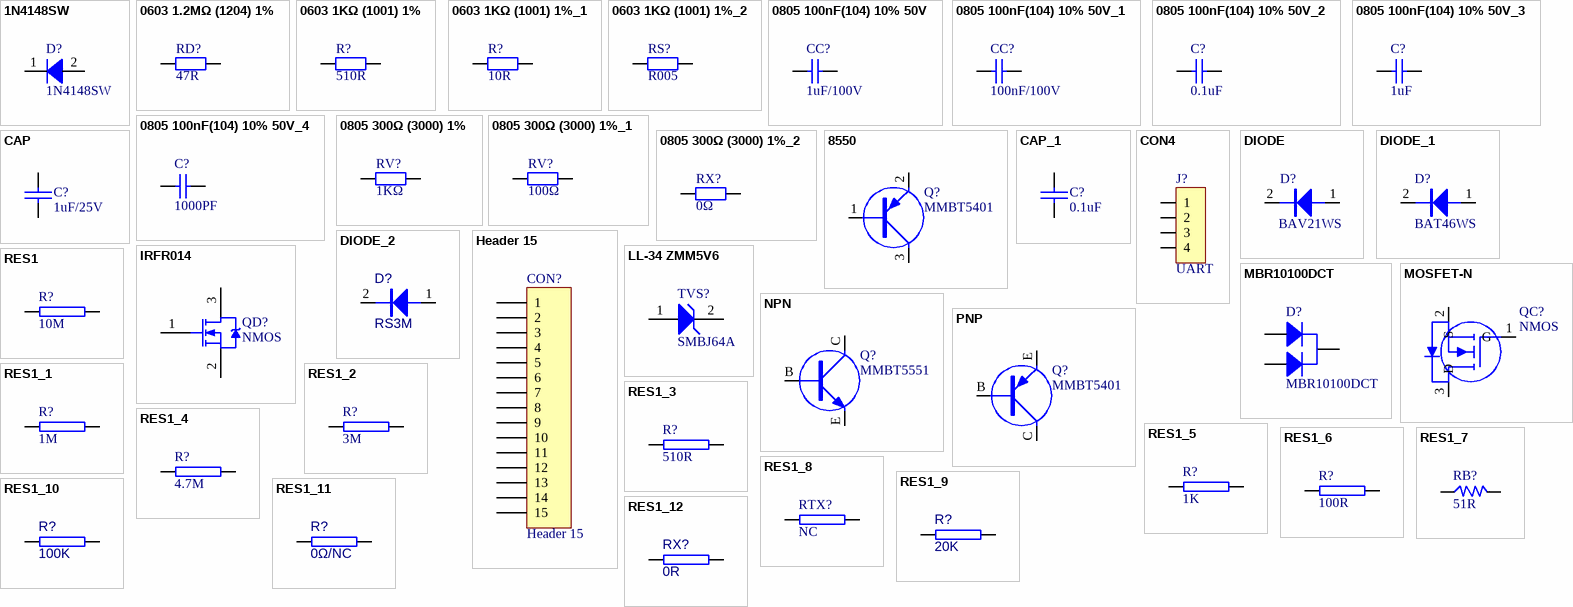
[diagram p0: symbols 1N4148SW to RES1_12]
# Altium schematic symbol library MISC84412-4.SchLib: 47 symbols
Pins are listed as number, name and electrical type; pins without a type are passive.


## 1N4148SW
designator D?
SMD diode
footprint SOD123 (SMD diode)
footprint SOD323 (SMD diode)
pins: 1 A, 2    

## 0603 1.2MΩ (1204) 1%
designator RD?, comment 47R
SMD resistor
footprint RES0603 (CAP0402)
footprint R0603A (SMD resistor)
footprint R0603Ap (SMD resistor)
pins: 1, 2
2 alternate drawings of the same symbol

## 0603 1KΩ (1001) 1%
designator R?, comment 510R
SMD resistor
footprint RES0603 (CAP0402)
footprint R0603A (SMD resistor)
footprint R0402L (SMD resistor)
footprint R0402A (SMD resistor)
pins: 1, 2
2 alternate drawings of the same symbol

## 0603 1KΩ (1001) 1%_1
designator R?, comment 10R
SMD resistor
footprint RES0603 (CAP0402)
footprint R0603A (SMD resistor)
footprint C0402A (SMD capacitor)
footprint R0402A (SMD resistor)
pins: 1, 2
2 alternate drawings of the same symbol

## 0603 1KΩ (1001) 1%_2
designator RS?, comment R005
SMD resistor
footprint 2512
footprint R2512L (SMD resistor)
pins: 1, 2
2 alternate drawings of the same symbol

## 0805 100nF(104) 10% 50V
designator CC?, comment 1uF/100V
SMD capacitor
footprint CAP0805
footprint C0805L (SMD capacitor)
pins: 1, 2
2 alternate drawings of the same symbol

## 0805 100nF(104) 10% 50V_1
designator CC?, comment 100nF/100V
SMD capacitor
footprint CAP0805
footprint C0603L (SMD J capacitor)
footprint C0805A (SMD capacitor)
footprint C0603A (SMD capacitor)
pins: 1, 2
2 alternate drawings of the same symbol

## 0805 100nF(104) 10% 50V_2
designator C?, comment 0.1uF
SMD capacitor
footprint CAP0603 (CAP0402)
footprint C0603A (SMD capacitor)
footprint C0402L (SMD resistor)
footprint C0402A (SMD capacitor)
pins: 1, 2
2 alternate drawings of the same symbol

## 0805 100nF(104) 10% 50V_3
designator C?, comment 1uF
SMD capacitor
footprint CAP0603 (CAP0402)
footprint C0603A (SMD capacitor)
footprint C0402L (SMD resistor)
footprint C0402A (SMD capacitor)
footprint C0402A (SMD capacitor)
pins: 1, 2
2 alternate drawings of the same symbol

## 0805 100nF(104) 10% 50V_4
designator C?, comment 1000PF
SMD capacitor
footprint CAP0603 (CAP0402)
footprint C0603A (SMD capacitor)
footprint C0402A (SMD capacitor)
pins: 1, 2
2 alternate drawings of the same symbol

## 0805 300Ω (3000) 1%
designator RV?, comment 1KΩ
SMD resistor
footprint RES0805
footprint R0805L (SMD resistor)
pins: 1, 2
2 alternate drawings of the same symbol

## 0805 300Ω (3000) 1%_1
designator RV?, comment 100Ω
SMD resistor
footprint RES0805
footprint R0805L (SMD resistor)
pins: 1, 2
2 alternate drawings of the same symbol

## 0805 300Ω (3000) 1%_2
designator RX?, comment 0Ω
SMD resistor
footprint RES0805
footprint R0805L (SMD resistor)
pins: 1, 2
2 alternate drawings of the same symbol

## 8550
designator Q?, comment MMBT5401
PNP
footprint SOT-23-3
footprint SOT23-3 (SMD IC/MOS*)
pins: 1, 2, 3

## CAP
designator C?, comment 1uF/25V
CAP
footprint 0603
footprint CAP0603 (CAP0402)
footprint C0603A (SMD capacitor)
pins: 1, 2

## CAP_1
designator C?, comment 0.1uF
CAP
footprint 0603
footprint CAP0603 (CAP0402)
footprint C0603
footprint C0603A (SMD capacitor)
pins: 1, 2

## CON4
designator J?, comment UART
footprint SIP-4
footprint CH-2.0-4P (Test socket 2.0mm)
pins: 1, 2, 3, 4

## DIODE
designator D?, comment BAV21WS
DIODE
footprint SOD323
footprint DIODE0.1
footprint DIODE0.3
footprint DIODE0.5
footprint SOD323(1+2-) (SMD diode)
pins: 1 A, 2 K
2 alternate drawings of the same symbol

## DIODE_1
designator D?, comment BAT46WS
DIODE
footprint SOD323
footprint DIODE0.1
footprint DIODE0.3
footprint DIODE0.5
footprint SOD323-T1 (SMD diode)
footprint SOD323(1+2-) (SMD diode)
pins: 1 A, 2 K
2 alternate drawings of the same symbol

## DIODE_2
designator D?, comment RS3M
DIODE
footprint DIODE0.4
footprint DIODE0.1
footprint DIODE0.3
footprint DIODE0.5
footprint SOD323
footprint SMC
footprint SMC
footprint SMB M(1+2-) (SMD diode)
pins: 1 A, 2 K
2 alternate drawings of the same symbol

## Header 15
designator CON?
Header15
footprint SIP-15-2.0-W
footprint PH-2.0mm15P弯脚不带扣 (PH-2.0mm15P right-angle connector, no latch)
pins: 1, 2, 3, 4, 5, 6, 7, 8, 9, 10, 11, 12, 13, 14, 15

## IRFR014
designator QD?, comment NMOS
HEXFET N-Channel Power MOSFET; Note: Pin 2 is trimmed and is electrically connected to Drain.; Value: 60V75A@0.94
footprint TO-252AA
footprint TO-263
footprint TOLL
pins: 1 G, 2 S, 3 D
2 alternate drawings of the same symbol

## LL-34 ZMM5V6
designator TVS?, comment SMBJ64A
Zener diode
footprint SOD123
footprint SMB A (1+2-) (SMD diode)
footprint SMB M(1+2-) (SMD diode)
footprint SMB M(1+2-) (SMD diode)
pins: 1 A, 2 K
2 alternate drawings of the same symbol

## MBR10100DCT
designator D?
SMD dual diode, common cathode
footprint TO-252-DIODE-DUAL (SMD diode)
pins: 1 A, 2 A, 3 K

## MOSFET-N
designator QC?, comment NMOS
footprint TO-252-A
footprint TO-252-DFN
pins: 1 G, 2 S, 3 D

## NPN
designator Q?, comment MMBT5551
NPN Transistor
footprint SOT-23
footprint SOT-23S
footprint SOT-23S
footprint SOT-23S
footprint SOT23-3 (SMD IC/MOS*)
footprint SOT23-3_BEC (SMD IC/MOS*)
pins: B, C, E
2 alternate drawings of the same symbol

## PNP
designator Q?, comment MMBT5401
PNP Transistor
footprint SOT-23S
footprint SOT-23S
footprint SOT23-3 (SMD IC/MOS*)
footprint SOT23-3_BEC (SMD IC/MOS*)
pins: B, C, E
2 alternate drawings of the same symbol

## RES1
designator R?, comment 10M
RES
footprint 0603
footprint RES0603 (CAP0402)
footprint R0603A (SMD resistor)
footprint C0402A (SMD capacitor)
footprint R0402A (SMD resistor)
pins: 1, 2

## RES1_1
designator R?, comment 1M
RES
footprint 0603
footprint RES0603 (CAP0402)
footprint R0603A (SMD resistor)
pins: 1, 2

## RES1_2
designator R?, comment 3M
RES
footprint 0603
footprint RES0603 (CAP0402)
footprint R0603A (SMD resistor)
pins: 1, 2

## RES1_3
designator R?, comment 510R
RES
footprint 0603
footprint RES0603 (CAP0402)
footprint R0603A (SMD resistor)
pins: 1, 2

## RES1_4
designator R?, comment 4.7M
RES
footprint 0603
footprint RES0603 (CAP0402)
footprint R0603A (SMD resistor)
pins: 1, 2

## RES1_5
designator R?, comment 1K
RES
footprint 0603
footprint RES0603 (CAP0402)
footprint R0603A (SMD resistor)
pins: 1, 2

## RES1_6
designator R?, comment 100R
RES
footprint 0603
footprint RES0603 (CAP0402)
footprint R0603A (SMD resistor)
footprint R0402A (SMD resistor)
pins: 1, 2

## RES1_7
designator RB?, comment 51R
±5% /UniOhm/yageo/TA-I/Walsin/Ralec
footprint R0603
footprint R0402
footprint R0805
footprint R1206 (1K±5% /1206/YAGEO)
footprint R1210
footprint R1812
footprint R2512
footprint 0201
footprint R2512-RS
footprint R1206
footprint RES0805
footprint R0805L (SMD resistor)
pins: 1, 2
2 alternate drawings of the same symbol

## RES1_8
designator RTX?, comment NC
RES
footprint 0603
footprint RES0603 (CAP0402)
footprint R0603A (SMD resistor)
pins: 1, 2

## RES1_9
designator R?, comment 20K
RES
footprint AXIAL0.3
footprint AXIAL0.4
footprint AXIAL0.5
footprint AXIAL0.6
footprint AXIAL0.8
footprint AXIAL0.8-2
footprint AXIAL1.2
footprint AXIAL1.2-2
footprint 0402
footprint 0603
footprint 0805
footprint RES0603 (CAP0402)
footprint R0603
footprint R0603A (SMD resistor)
pins: 1, 2

## RES1_10
designator R?, comment 100K
RES
footprint AXIAL0.3
footprint AXIAL0.4
footprint AXIAL0.5
footprint AXIAL0.6
footprint AXIAL0.8
footprint AXIAL0.8-2
footprint AXIAL1.2
footprint AXIAL1.2-2
footprint 0402
footprint 0603
footprint 0805
footprint RES0603 (CAP0402)
footprint R0603
footprint R0603A (SMD resistor)
pins: 1, 2

## RES1_11
designator R?, comment 0Ω/NC
RES
footprint AXIAL0.3
footprint AXIAL0.4
footprint AXIAL0.5
footprint AXIAL0.6
footprint AXIAL0.8
footprint AXIAL0.8-2
footprint AXIAL1.2
footprint AXIAL1.2-2
footprint 0402
footprint 0603
footprint 0805
footprint RES0603 (CAP0402)
footprint R0603
footprint R0603A (SMD resistor)
pins: 1, 2

## RES1_12
designator RX?, comment 0R
RES
footprint AXIAL0.3
footprint AXIAL0.4
footprint AXIAL0.5
footprint AXIAL0.6
footprint AXIAL0.8
footprint AXIAL0.8-2
footprint AXIAL1.2
footprint AXIAL1.2-2
footprint 0402
footprint 0603
footprint 0805
footprint RES0603 (CAP0402)
footprint R0603
footprint R0603A (SMD resistor)
pins: 1, 2

## RES2
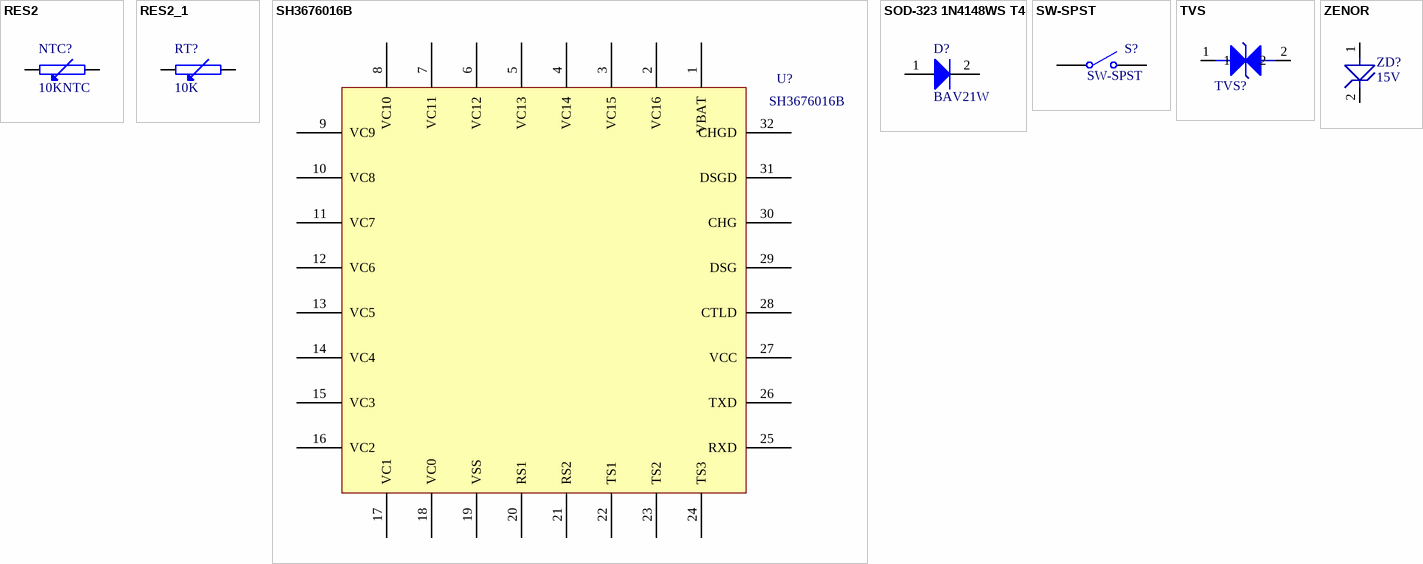
[diagram p1: symbols RES2 to ZENOR]
## RES2
designator NTC?, comment 10KNTC
RES
footprint WK
footprint RT2.3X1-2 (Wire-soldered NTC)
pins: 1, 2
2 alternate drawings of the same symbol

## RES2_1
designator RT?, comment 10K
RES
footprint RES0603 (CAP0402)
footprint R0603A (SMD resistor)
pins: 1, 2
2 alternate drawings of the same symbol

## SH3676016B
designator U?
footprint LQFP32
footprint LQFP32
footprint LQFP32L(pin间距0.5mm) (SMD IC)
footprint LQFP32L(PIN间距0.8mm) (SMD IC (Sino Wealth SH3676014/16BP))
pins: 1 VBAT, 2 VC16, 3 VC15, 4 VC14, 5 VC13, 6 VC12, 7 VC11, 8 VC10, 9 VC9, 10 VC8, 11 VC7, 12 VC6, 13 VC5, 14 VC4, 15 VC3, 16 VC2, 17 VC1, 18 VC0, 19 VSS, 20 RS1, 21 RS2, 22 TS1, 23 TS2, 24 TS3, 25 RXD, 26 TXD, 27 VCC, 28 CTLD, 29 DSG, 30 CHG, 31 DSGD, 32 CHGD
2 alternate drawings of the same symbol

## SOD-323 1N4148WS T4
designator D?, comment BAV21W
Diode
footprint SOD123
footprint SOD123
footprint SOD323(1+2-) (SMD diode)
pins: 1 A, 2 K
2 alternate drawings of the same symbol

## SW-SPST
designator S?
Single-Pole, Single-Throw Switch
footprint WK
footprint NTC-DIP
footprint RT2.3X1.2-2 (Wire-soldered NTC)
pins: 1 COMMON, 2 NO

## TVS
designator TVS?, comment 75CA  (value not drawn)
TVS
footprint SMA
footprint SMC (DO-214-AB/SMC; 2 C-Bend Leads; Body 7.9 x 5.9 mm, inc. leads (LxW))
footprint SMC A-TVS(DO-214AB) (SMD diode)
footprint SMC_M(DO-214AB) (SMD diode)
pins: 1, 2
2 alternate drawings of the same symbol

## ZENOR
designator ZD?, comment 15V
ZENOR
footprint SOD323
footprint SOD323(1+2-) (SMD diode)
footprint C0402A (SMD capacitor)
pins: 1, 2
2 alternate drawings of the same symbol